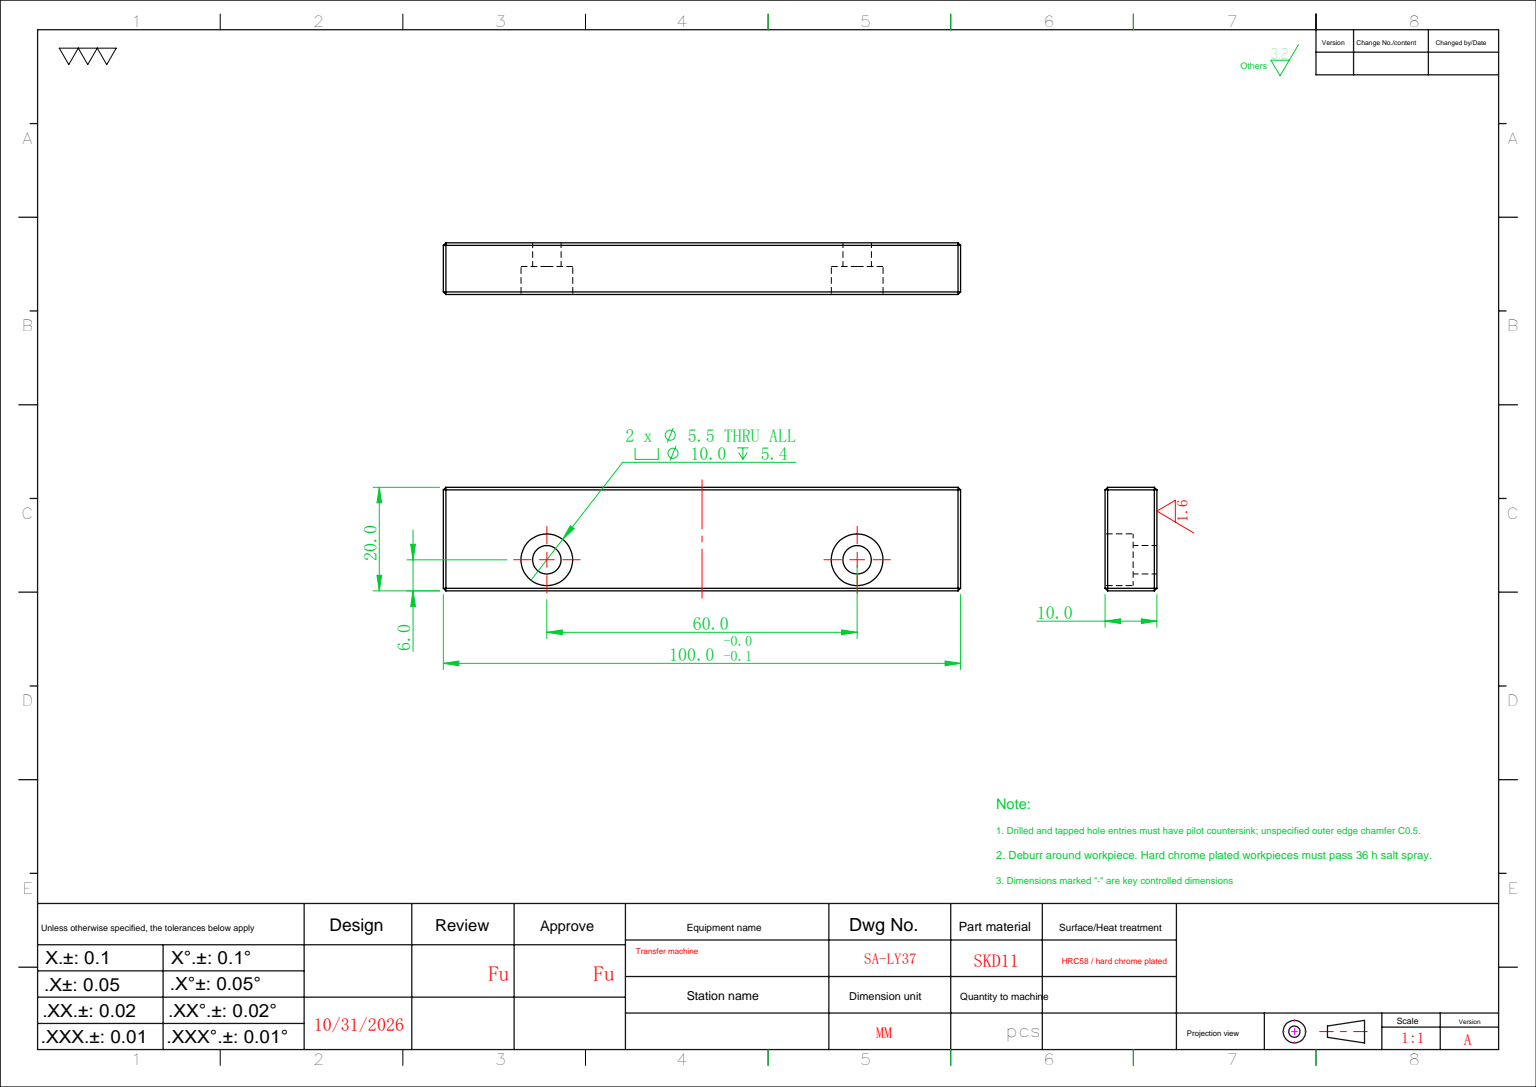
from build123d import *

# Parameters (mm, degrees)
SKETCH_1_W                   = 10
SKETCH_1_H                   = 100
EXTRUDE_1_DEPTH              = 20
HOLE_WIZARD_M5_1_D           = 5.5
HOLE_WIZARD_M5_1_CBORE_D     = 10
HOLE_WIZARD_M5_1_CBORE_DEPTH = 5.4
CHAMFER_1_SIZE               = 0.5


with BuildPart() as part:
    # 草图1 → 凸台-拉伸1 (new body)
    with BuildSketch(Plane.XY):
        Rectangle(SKETCH_1_W, SKETCH_1_H)
    extrude(amount=EXTRUDE_1_DEPTH)

    # M5 六角凹头螺钉的柱形沉头孔1 (through all)
    with Locations(Plane.ZY.offset(5)):
        with Locations((6, 30), (6, -30)):
            CounterBoreHole(HOLE_WIZARD_M5_1_D / 2, HOLE_WIZARD_M5_1_CBORE_D / 2, HOLE_WIZARD_M5_1_CBORE_DEPTH)

    # 倒角1
    chamfer_1_edges = [part.edges().sort_by_distance(p)[0] for p in [
        (-5, 0, 20),
        (0, -50, 20),
        (5, 0, 20),
        (0, -50, 0),
        (-5, 0, 0),
        (0, 50, 0),
        (5, 0, 0),
        (5, -50, 10),
        (-5, -50, 10),
        (-5, 50, 10),
        (5, 50, 10),
        (0, 50, 20),
    ]]
    chamfer(chamfer_1_edges, length=CHAMFER_1_SIZE)


solid = part.part
